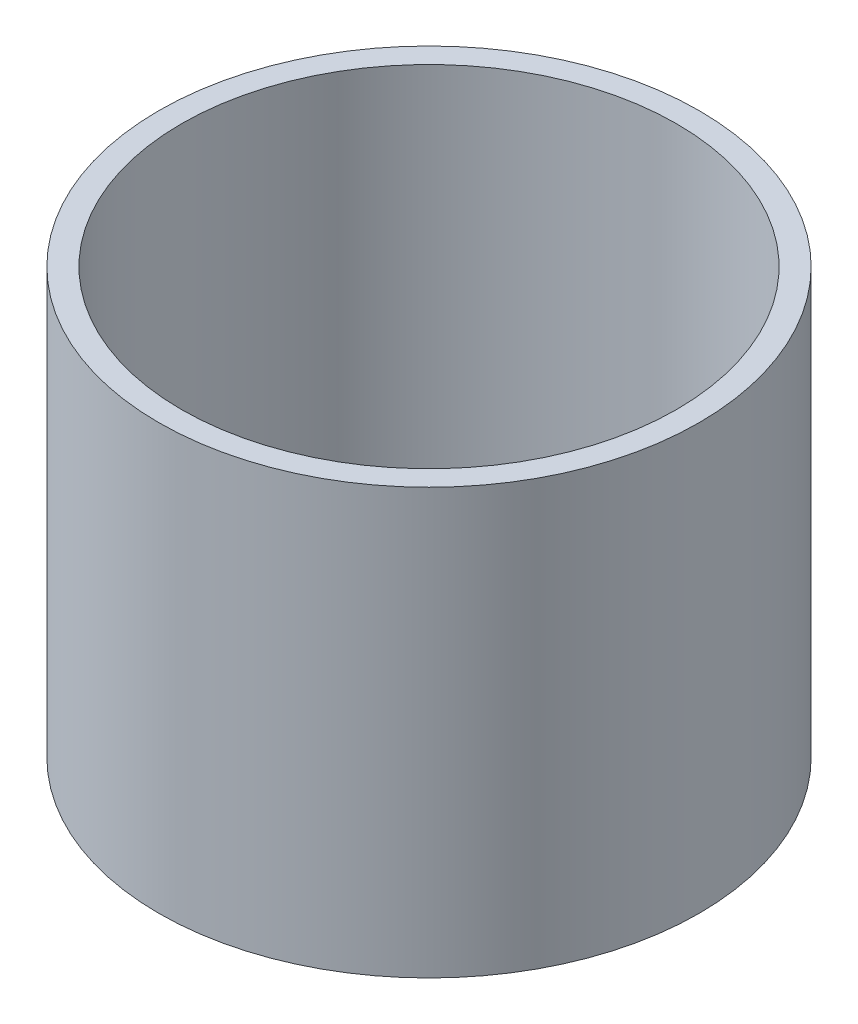
from build123d import *

# Parameters (mm, degrees)
SKETCH1_R           = 38.15
SKETCH1_R_2         = 34.95
BOSS_EXTRUDE1_DEPTH = 60


with BuildPart() as part:
    # Sketch1 → Boss-Extrude1 (new body)
    with BuildSketch(Plane(origin=(0, 0, 0), x_dir=(1, 0, 0), z_dir=(0, 1, 0))):
        with Locations(Location((0, 0, 0), (0, 0, 270))):
            Circle(SKETCH1_R)
        with Locations(Location((0, 0, 0), (0, 0, 270))):
            Circle(SKETCH1_R_2, mode=Mode.SUBTRACT)
    extrude(amount=BOSS_EXTRUDE1_DEPTH)


solid = part.part
